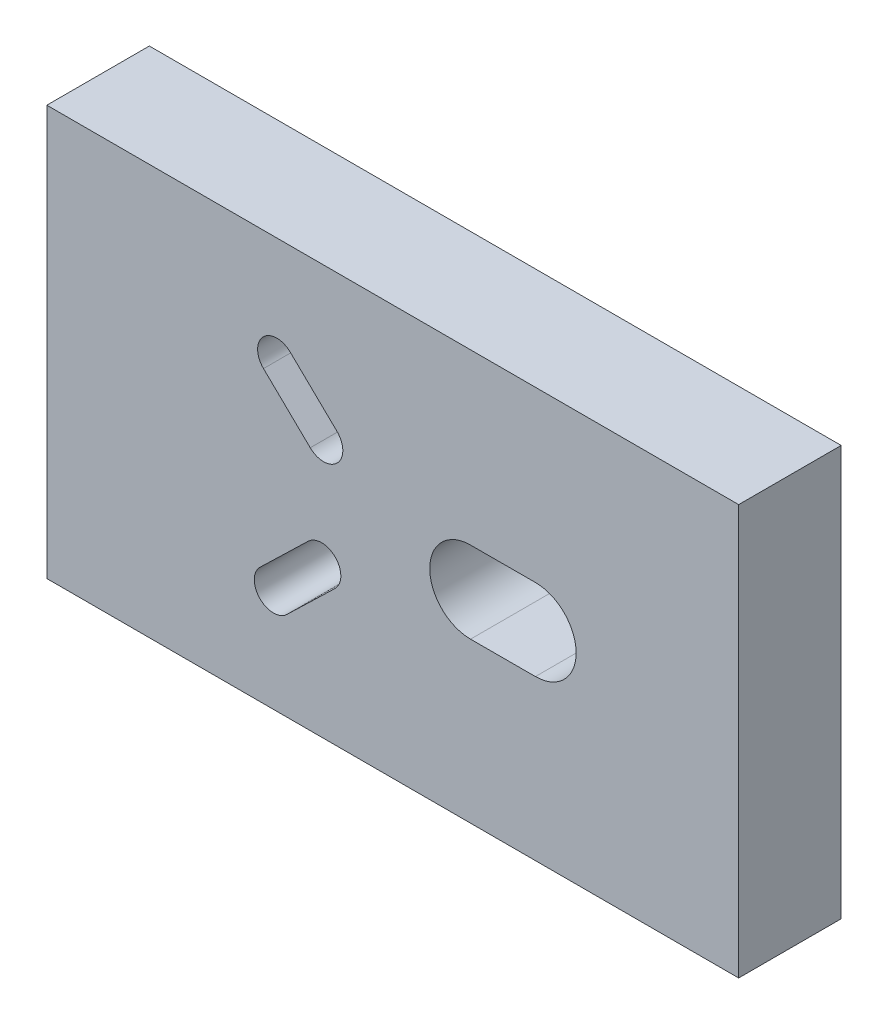
from build123d import *

# Parameters (mm, degrees)
SKETCH_1_W          = 27
SKETCH_1_H          = 16
EXTRUDE_1_DEPTH     = 4
SKETCH_2_R          = 0.75
SKETCH_2_R_2        = 1.59
CUT_EXTRUDE_2_DEPTH = 4
CUT_EXTRUDE_3_DEPTH = 4


with BuildPart() as part:
    # 草图1 → 凸台-拉伸1 (new body)
    with BuildSketch(Plane.XY):
        with Locations((3.898916968, -3.881768953)):
            Rectangle(SKETCH_1_W, SKETCH_1_H)
    extrude(amount=EXTRUDE_1_DEPTH)

    # 草图2 → 切除-拉伸2 (cut)
    with BuildSketch(Plane.XY.offset(4)):
        with Locations((1.199905932, -1.781578746)):
            Circle(SKETCH_2_R)
        with Locations((1.122511443, -6.056778774)):
            Circle(SKETCH_2_R)
        with Locations((9.465404763, -4.069510677)):
            Circle(SKETCH_2_R_2)
    extrude(amount=-CUT_EXTRUDE_2_DEPTH, mode=Mode.SUBTRACT)

    # 草图3 → 切除-拉伸3 (cut)
    with BuildSketch(Plane.XY.offset(4)):
        with BuildLine():
            Line((6.931862452, -2.481455291), (9.464184068, -2.479511145))
            ThreePointArc((9.464184068, -2.479511145), (7.875405231, -4.070731371), (9.466625457, -5.659510208))
            Line((9.466625457, -5.659510208), (6.934303841, -5.661454354))
            ThreePointArc((6.934303841, -5.661454354), (5.343083615, -4.072675517), (6.931862452, -2.481455291))
        make_face()
        with BuildLine():
            Line((-1.276445305, -7.332757851), (0.601227077, -5.517554692))
            ThreePointArc((0.601227077, -5.517554692), (0.583287361, -6.578063139), (1.643795809, -6.596002856))
            Line((1.643795809, -6.596002856), (-0.233876574, -8.411206015))
            ThreePointArc((-0.233876574, -8.411206015), (-1.294385021, -8.393266299), (-1.276445305, -7.332757851))
        make_face()
        with BuildLine():
            Line((-1.145979965, -0.556904877), (0.678621567, -2.320802827))
            ThreePointArc((0.678621567, -2.320802827), (0.660681851, -1.26029438), (1.721190298, -1.242354664))
            Line((1.721190298, -1.242354664), (-0.103411234, 0.521543286))
            ThreePointArc((-0.103411234, 0.521543286), (-1.163919681, 0.50360357), (-1.145979965, -0.556904877))
        make_face()
    extrude(amount=-CUT_EXTRUDE_3_DEPTH, mode=Mode.SUBTRACT)


solid = part.part
